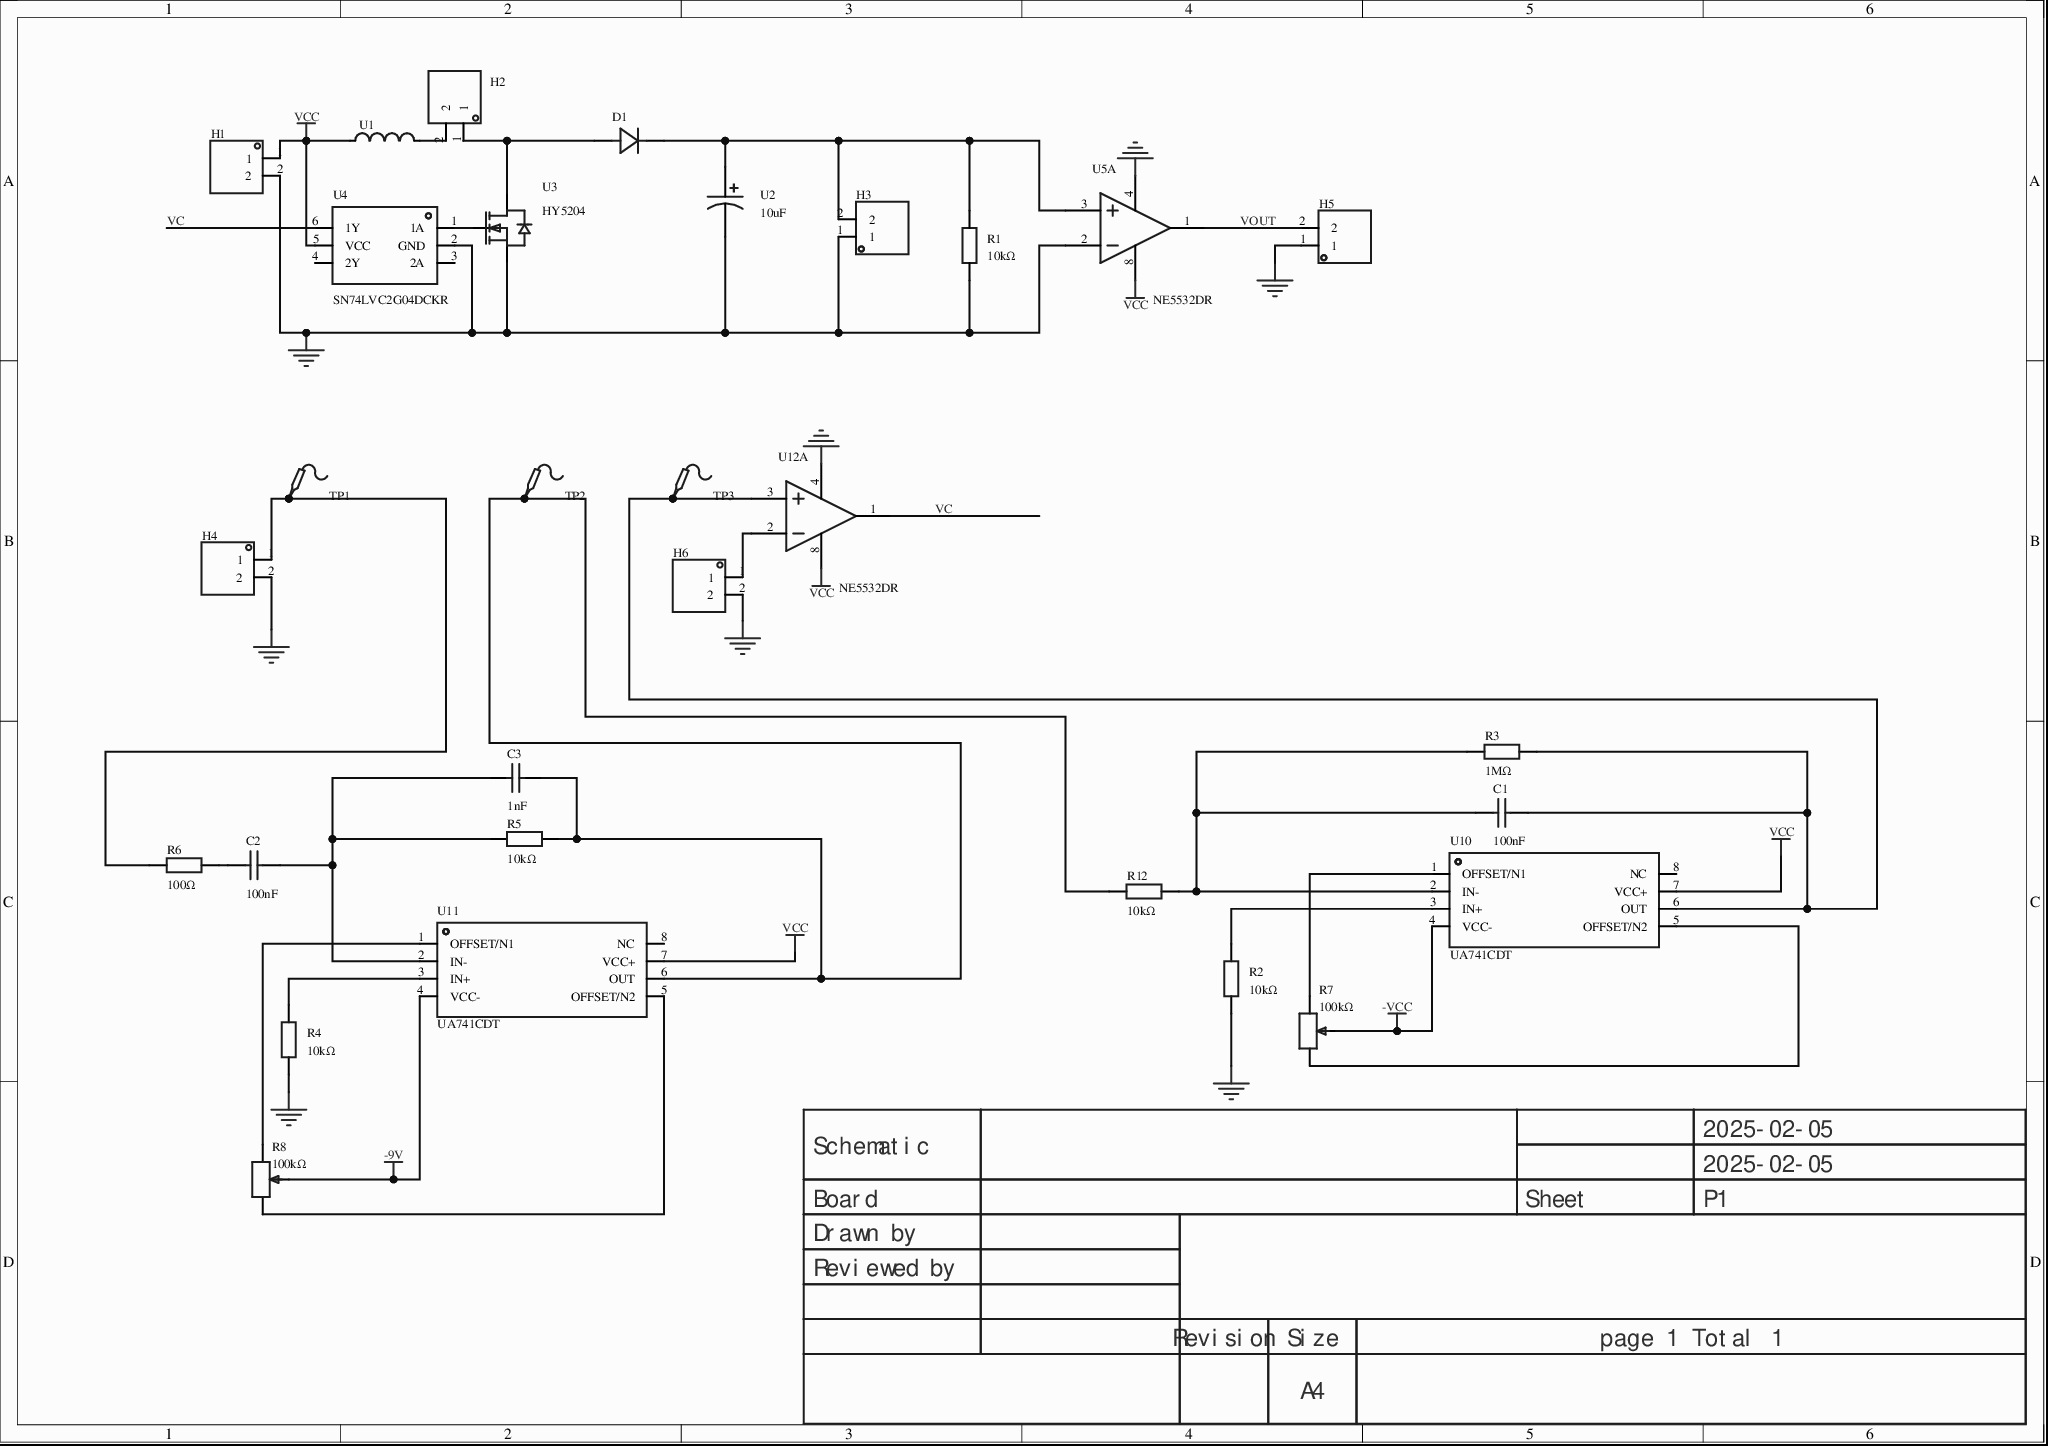
[diagram p0: MISC89040-3.schdoc]
# Altium project MISC89040-2.PrjPcb
1 sheet, 30 parts. Net scope: global (net labels, ports and power ports of the same name join across sheets).
Board file: MISC89040.pcbdoc

## Sheet MISC89040-3.schdoc
size 297 x 209 mm; Version: V1.0; @Project Name: MISC89040; @Page Count: 1; @Update Date: 2025-02-05; @Create Date: 2025-02-05; @Schematic Name: MISC89040; @Page No: 1; @Create Time: 14:09:58; @Update Time: 15:16:38; @Board Name: MISC89040

### Parts
C1  100nF  [C0805]
C2  100nF  [C0805]
C3  1nF  [C0805]
D1  (no value)  [DO_1N4007]
H1  (no value)  [HDR-TH_2P-P2.54-V-M-1]
H2  (no value)  [HDR-TH_2P-P2.54-V-M-1]
H3  (no value)  [HDR-TH_2P-P2.54-V-M-1]
H4  (no value)  [HDR-TH_2P-P2.54-V-M-1]
H5  (no value)  [HDR-TH_2P-P2.54-V-M-1]
H6  (no value)  [HDR-TH_2P-P2.54-V-M-1]
R1  10kΩ  [Res_1/4W]
R2  10kΩ  [R0805]
R3  1MΩ  [R0805]
R4  10kΩ  [R0805]
R5  10kΩ  [R0805]
R6  100Ω  [R0805]
R7  100kΩ  [RES-ADJ-SMD_VG039NCH]
R8  100kΩ  [RES-ADJ-SMD_VG039NCH]
R12  10kΩ  [R0805]
TP1  (no value)  [Test-Point-0.5mm]
TP2  (no value)  [Test-Point-0.5mm]
TP3  (no value)  [Test-Point-0.5mm]
U1  Power inductor (SMD),CKST0502-10uH/M,10uH,±20%,3A,package 5.7mm*5.1mm*2.0mm,CENKER,RoHS  [IND-SMD_L5.7-W5.1]  (value not drawn)
U2  10uF  [CAP-TH_BD4.0-P1.50-D0.8-FD]
U3  HY5204  [TO-247-3_L15.8-W5.0-P5.44-L-1]
U4  SN74LVC2G04DCKR  [SOT-363_L2.0-W1.3-P0.65-LS2.1-BR]
U5  NE5532DR  [SOIC-8_L4.9-W3.9-P1.27-LS6.0-BL]  (part A of 2)
U10  UA741CDT  [SOIC-8_L4.9-W3.9-P1.27-LS6.0-BL]
U11  UA741CDT  [SOIC-8_L4.9-W3.9-P1.27-LS6.0-BL]
U12  NE5532DR  [SOIC-8_L4.9-W3.9-P1.27-LS6.0-BL]  (part A of 2)

### Nets
-9V: R8.2 U11.4(VCC-)
-VCC: R7.2 U10.4(VCC-)
GND: H1.2 H3.1 H4.2 H5.1 H6.2 R1.1 R2.1 R4.1 U2.2 U3.3(S) U4.2(GND) U5.2(IN1-) U5.4(VCC-/GND) U12.4(VCC-/GND)
VCC: H1.1 U1.1 U4.5(VCC) U5.8(VCC+) U10.7(VCC+) U11.7(VCC+) U12.8(VCC+)
VC: U4.6(1Y) U12.1(OUT1)
VOUT: H5.2 U5.1(OUT1)
NetC1_1: C1.1 R3.1 R12.2 U10.2(IN-)
NetC1_2: C1.2 R3.2 TP3.1 U10.6(OUT) U12.3(IN1+)
NetC2_1: C2.1 R6.2
NetC2_2: C2.2 C3.1 R5.1 U11.2(IN-)
NetC3_2: C3.2 R5.2 R12.1 TP2.1 U11.6(OUT)
NetD1_1: D1.1(K) H3.2 R1.2 U2.1 U5.3(IN1+)
NetD1_2: D1.2(A) H2.1 U3.2(D)
NetH2_2: H2.2 U1.2
NetH4_1: H4.1 R6.1 TP1.1
NetH6_1: H6.1 U12.2(IN1-)
NetR2_2: R2.2 U10.3(IN+)
NetR4_2: R4.2 U11.3(IN+)
NetR7_1: R7.1 U10.5(OFFSET/N2)
NetR7_3: R7.3 U10.1(OFFSET/N1)
NetR8_1: R8.1 U11.1(OFFSET/N1)
NetR8_3: R8.3 U11.5(OFFSET/N2)
NetU3_1: U3.1(G) U4.1(1A)

Not connected (* = marked no-connect by the designer): U4 3(2A)* 4(2Y)*; U10 8(NC); U11 8(NC)

### Notes on the sheet
- 2025-02-05
- Schematic
- Board
- Sheet
- P1
- Drawn by
- Reviewed by
- Revision
- Size
- A4
- page 1 Total 1

### Library data of the parts
C1-C3 = CC0805KRX7R9BB104: Capacitance:100nF;Tolerance:±10%;Rated voltage:50V;Material (temperature coefficient):X7R;; Manufacturer: YAGEO(国巨); AddInBom: yes; ModelId: 1ba041120af144c991958decab20d241; ModelName: C0805_L2.0-W1.3-H1.3; ModelTransform: 78.74,51.181,0,0,0,0,0,0.0005,0; Tolerance: ±10%; Voltage Rated: 50V; Temperature Coefficient: X7R; Symbol: CC0805KRX7R9BB104; Device: CC0805KRX7R9BB104; LCSC Part Name: 100nF ±10% 50V; ManufacturerPart: CC0805KRX7R9BB104; Supplier Footprint: 0805; JLCPCB Part Class: Basic library; Datasheet: https://atta.szlcsc.com/upload/public/pdf/source/20180224/C181747_15194369449651363981.pdf; Supplier: LCSC; ConvertToPcb: yes; FootprintName: C0805
  C1 C2: SupplierPart: C49678; Value: 100nF
  C3: Value: 1nF
D1 = D_1N4007A: AddInBom: yes; ModelId: 6de1e9b71a0d4751b4e9df530304c1a3; ModelName: DO-41_D2.4-L4.7-P8.70; ModelTransform: 373.9,94.4,232.29,0,0,0,0,0,-140; Symbol: D_1N4007; Device: D_1N4007A; Supplier Footprint: DO-41; ConvertToPcb: yes; FootprintName: DO_1N4007
H1-H6 = HDR-M_2.54_1x2P: Symbol: 210S-1*2P L=11.6MMGold-plated black; ConvertToPcb: yes; ModelId: 79b2e9f2d70a4d68a1b7098f27c6d4c5; ModelName: HDR-M-2.54_1x2; ModelTransform: 200,100,0,0,0,0,0,0,-118.11; Device: HDR-M_2.54_1x2P; AddInBom: yes; SupplierPart: C124375; Supplier Footprint: 插件; FootprintName: HDR-TH_2P-P2.54-V-M-1
R1 = Res_AXIAL-1/4W: AddInBom: yes; SymbolName: Resistor; ModelId: 463263665006444ab7a47bd11b0cf956; ModelName: RES-TH_BD2.4-L6.3-P10.30-D0.6; ModelTransform: 427.165,94.32816,0,0,0,0,0,0,-196.85; Device: Res_AXIAL-1/4W; Supplier Footprint: 轴向引线; ConvertToPcb: yes; FootprintName: Res_1/4W; Value: 10kΩ
R2-R6 R12 = 0805W8F1002T5E_C17414: Resistor type:Thick film resistor;Resistance:10kΩ;Tolerance:±1%;Power:125mW;Max working voltage:150V;Temperature coefficient:±100ppm/℃;; Manufacturer: UNI-ROYAL(厚声); AddInBom: yes; ModelId: 37a81e68749a4138bd2dfa6897b24b85; ModelName: R0805_L2.0-W1.3-H0.6; ModelTransform: 78.74,51.181,0,0,0,0,0,-0.0005,0; Tolerance: ±1%; Power(Watts): 125mW; Overload Voltage (Max): 150V; Symbol: 0805W8F1002T5E; Device: 0805W8F1002T5E_C17414; Supplier: LCSC; Manufacturer Part: 0805W8F1002T5E; JLCPCB Part Class: Basic library; LCSC Part Name: 10kΩ ±1% 125mW 厚膜电阻; Supplier Footprint: 0805; Datasheet: https://atta.szlcsc.com/upload/public/pdf/source/20200306/C422600_1E6D84923E4A46A82E41ADD87F860B5C.pdf; ConvertToPcb: yes; FootprintName: R0805; Type: Thick film resistor; Temperature Coefficient: ±100ppm/℃; Operating Temperature Range: -55℃~+155℃
  R2 R4 R5 R12: Supplier Part: C17414; Value: 10kΩ
  R3: Value: 1MΩ
  R6: Value: 100Ω
R7 R8 = VG039NCHXTB201: Resistance:200Ω;Tolerance:±25%;; Manufacturer: HDK(北陆电气); AddInBom: yes; ModelId: ba438d2707b74a9ab8400a10f68363a0; ModelName: RES-ADJ-SMD_3P-L3.8-W3.0-H1.2-P1.90; ModelTransform: 120.0785,161.61385,0,90,0,0,-3.74,-0.118,0; Tolerance: ±25%; Value: 100kΩ; Device: VG039NCHXTB201; Symbol: VG039NCHXTB201; LCSC Part Name: 200Ω ±25%; ManufacturerPart: VG039NCHXTB201; Supplier Footprint: SMD; JLCPCB Part Class: Extended library; Datasheet: https://atta.szlcsc.com/upload/public/pdf/source/20171123/C145162_15114111014461137838.pdf; Supplier: LCSC; ConvertToPcb: yes; FootprintName: RES-ADJ-SMD_VG039NCH
TP1-TP3 = Test-Point: Test Point; AddInBom: yes; Device: Test-Point; ConvertToPcb: yes; SymbolName: Test-Point; FootprintName: Test-Point-0.5mm
U1 = 功率电感(贴片),CKST0502-10uH/M,10uH,±20%,3A,封装5.7mm*5.1mm*2.0mm,岑科,RoHS: AddInBom: yes; ModelId: ffd856615f974dd9b1ff3f65e3b3100d; ModelTransform: 224.409,200.787,0,0,0,0,0,-0.591,0; Symbol: Power inductor (SMD),CKST0502-10UH/M,10UH,±20%,3A,package 5.7MM*5.1MM*2.0MM,CENKER,ROHS; Device: Power inductor (SMD),CKST0502-10uH/M,10uH,±20%,3A,package 5.7mm*5.1mm*2.0mm,CENKER,RoHS; LCSC Part Name: 功率电感(贴片),CKST0502-10uH/M,10uH,±20%,3A,封装5.7mm*5.1mm*2.0mm,岑科,RoHS; SupplierPart: C9900015114; ManufacturerPart: 功率电感(贴片),CKST0502-10uH/M,10uH,±20%,3A,封装5.7mm*5.1mm*2.0mm,岑科,RoHS; Supplier Footprint: 功率电感(贴片),CKST0502-10uH/M,10uH,±20%,3A,封装5.7mm*5.1mm*2.0mm,岑科,RoHS; JLCPCB Part Class: Extended library; Supplier: LCSC; ConvertToPcb: yes; FootprintName: IND-SMD_L5.7-W5.1; ModelName: IND-SMD_L5.7-W5.1
U2 = 10MS510MEFC4X5: Capacitance:10uF;Tolerance:±20%;Rated voltage:10V;Ripple current:16mA@120Hz;; Manufacturer: rubycon(红宝石); AddInBom: yes; ModelId: 8017ea3dd4884afab5fc61dd7898abc1; ModelName: CAP-TH_D4.0-H7.0-P1.5; ModelTransform: 158.2674,157.45008,0,0,0,0,0,0,-137.795; Tolerance: ±20%; Rated Voltage: 10V; φD: 4mm; L: 5mm; Lifetime @ Temp: 1000hrs@85℃; Symbol: 10MS510MEFC4X5; Device: 10MS510MEFC4X5; LCSC Part Name: 10uF ±20% 10V; SupplierPart: C1579578; ManufacturerPart: 10MS510MEFC4X5; Supplier Footprint: 插件,D4xL5mm; JLCPCB Part Class: Extended library; Datasheet: https://atta.szlcsc.com/upload/public/pdf/source/20210510/C1579578_ABB61F9CFFB4E7371AD0DBD373B61F20.pdf; Supplier: LCSC; ConvertToPcb: yes; FootprintName: CAP-TH_BD4.0-P1.50-D0.8-FD; Value: 10uF; Ripple Current: 16mA@120Hz; Lead Spacing: 1.5mm; Operating Temperature: -40℃~+85℃
U3 = HY5204: AddInBom: yes; ModelId: 27b35664da8045b09b6c38d0310660f0; ModelTransform: 614.17235,196.88937,0,0,0,0,0,7.874,-196.85; Symbol: HY5204; Device: HY5204; LCSC Part Name: HY5204; SupplierPart: C9900006698; ManufacturerPart: HY5204; Supplier Footprint: MOSFET-N; JLCPCB Part Class: Extended library; Supplier: LCSC; ConvertToPcb: yes; FootprintName: TO-247-3_L15.8-W5.0-P5.44-L-1; ModelName: TO-247-3_L15.8-W5.0-P5.44-L-1
U4 = SN74LVC2G04DCKR: Input type:-;Supply voltage:1.65V~5.5V;Supply current (max):10uA;Number of circuits:2;Max propagation delay (tpd):3.2ns@5V,50pF;; Manufacturer: TI(德州仪器); AddInBom: yes; ModelId: ea15c7b026c54341854a7f0d9614aed9; ModelName: SOT-363-6P_L2.0-W1.3-H1.1-LS2.0-P0.65; ModelTransform: 83.17133,78.74,0,180,0,0,0,0,0; Supply Current (Max): 10uA; Number of Circuits: 2; Sink Current: 32mA; High level range (VIH): 1.7V~2V; Low level range (VIL): 700mV~800mV; Symbol: SN74LVC2G04DCKR; Device: SN74LVC2G04DCKR; LCSC Part Name: 双路反相器; SupplierPart: C105251; ManufacturerPart: SN74LVC2G04DCKR; Supplier Footprint: SOT-363-6; JLCPCB Part Class: Extended library; Supplier: LCSC; ConvertToPcb: yes; FootprintName: SOT-363_L2.0-W1.3-P0.65-LS2.1-BR; Input Type: -; Supply Voltage(Single): 1.65V~5.5V; Number of Inputs: 2; Source Current: 32mA; Max Propagation Delay: 3.2ns@5V,50pF; Series: 74LVC series; Operating Temperature: -40℃~+125℃
U5 U12 = NE5532DR: Number of amplifiers:Dual;Gain bandwidth product (GBP):10MHz;Input bias current (Ib):200nA;Slew rate (SR):9V/us;Bandwidth (-3db):-;; Manufacturer: TI(德州仪器); Relevance: []; AddInBom: yes; ModelId: e81d2f7d937b4a6ab1dca543ff5d56a4; ModelName: SOIC-8_L4.9-W3.9-H1.7-LS6.0-P1.27; ModelTransform: 189.751,236.22,0,0,0,0,0.0005,0.0005,0; Number of Circuits: Dual; Gain Bandwidth Product(GBP): 10MHz; Current - Input Bias(Ib): 200nA; Slew Rate(SR): 9V/us; Output Current: 38mA; Supply Current: 8mA; Symbol: NE5532DR; Device: NE5532DR; LCSC Part Name: NE5532DR; SupplierPart: C7426; ManufacturerPart: NE5532DR; Supplier Footprint: SOIC-8; Supplier: LCSC; ConvertToPcb: yes; FootprintName: SOIC-8_L4.9-W3.9-P1.27-LS6.0-BL; -3db Bandwidth: -; Operating Temperature: 0℃~+70℃
U10 U11 = UA741CDT: Number of amplifiers:Single;Gain bandwidth product (GBP):1MHz;Input bias current (Ib):10nA;Slew rate (SR):0.5V/us;Bandwidth (-3db):-;; Manufacturer: ST(意法半导体); AddInBom: yes; ModelId: e81d2f7d937b4a6ab1dca543ff5d56a4; ModelName: SOIC-8_L4.9-W3.9-H1.7-LS6.0-P1.27; ModelTransform: 189.751,236.22,0,0,0,0,0.0005,0.0005,0; Number of Circuits: Single; Gain Bandwidth Product(GBP): 1MHz; Current - Input Bias(Ib): 10nA; Output Current: 25mA; Supply Current: 3.3mA; Symbol: UA741CDT; Device: UA741CDT; LCSC Part Name: UA741CDT; SupplierPart: C7111; ManufacturerPart: UA741CDT; Supplier Footprint: SOIC-8; JLCPCB Part Class: Extended library; Datasheet: https://atta.szlcsc.com/upload/public/pdf/source/20181030/C283333_E7CFD90DFDEB0B09152BEF9966FA2369.pdf; Supplier: LCSC; ConvertToPcb: yes; FootprintName: SOIC-8_L4.9-W3.9-P1.27-LS6.0-BL; Slew Rate(SR): 0.5V/us; -3db Bandwidth: -; Operating Temperature: 0℃~+70℃